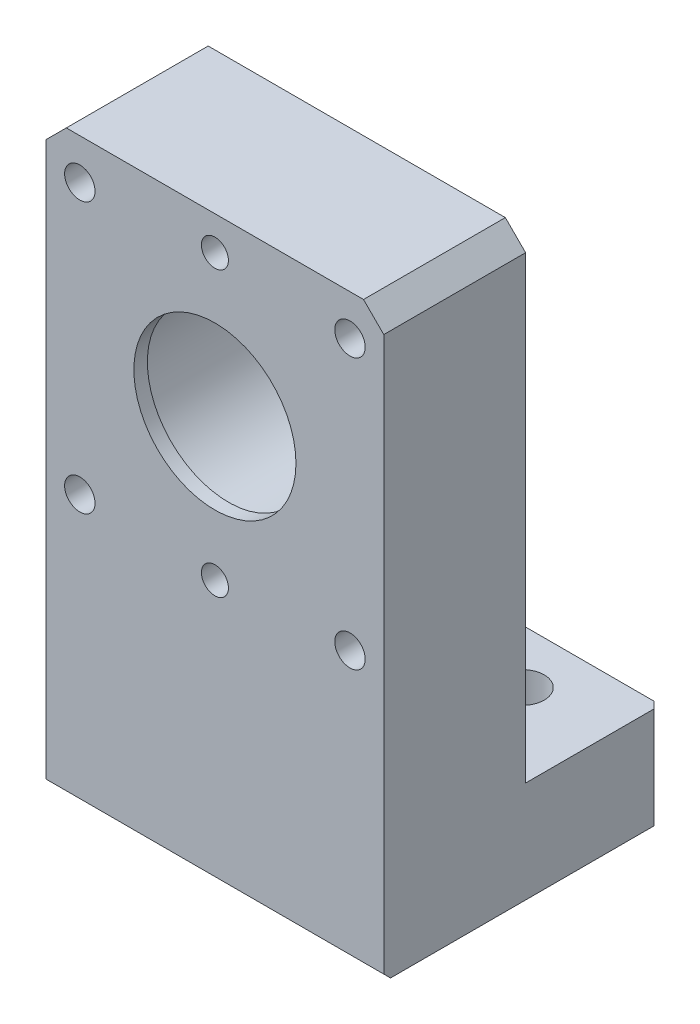
SolidWorks part; units mm, degrees
ref_plane "Front Plane" through (0, 0, 0) normal (0, 0, 1) x (1, 0, 0)
ref_plane "Top Plane" through (0, 0, 0) normal (0, 1, 0) x (1, 0, 0)
ref_plane "Right Plane" through (0, 0, 0) normal (1, 0, 0) x (0, 0, -1)
sketch "Sketch3" plane through (0, 0, 0) normal (0, 0, 1) x (1, 0, 0)
  line L1 (25, 0) -> (-25, 0)
  line L2 (25, 0) -> (25, 86)
  line L3 (25, 86) -> (-25, 86)
  line L4 (-25, 0) -> (-25, 86)
  circle A0 centre (0, 60) radius 14
  dimension "D3" = 28
  dimension "D4" = 60
  dimension "D1" = 50
  dimension "D2" = 86
extrude "Boss-Extrude1" add sketch "Sketch3" along normal blind 21
sketch "Sketch4" plane through (0, 0, 21) normal (0, 0, 1) x (1, 0, 0)
  circle A0 centre (0, 60) radius 14
  circle A1 centre (0, 60) radius 12
  dimension "D1" = 28
  dimension "D2" = 24
hole_wizard "M3 Tapped Hole1" positions "Sketch7" profile "Sketch6" tap size "M3" standard "GB"
sketch "Sketch7" plane through (6.3989, 17.9257, 0) normal (0, 0, 1) x (1, 0, 0)
  line L2 (-6.3989, 42.0743) -> (11.6011, 42.0743) construction
  line L4 (-6.3989, 42.0743) -> (-24.3989, 42.0743) construction
  point P0 (11.6011, 42.0743)
  point P1 (-24.3989, 42.0743)
  dimension "D1" = 18
  dimension "D2" = 18
sketch "Sketch6" plane through (18, 60, 0) normal (1, 0, 0) x (0, 1, 0)
  line L0 (0, 0) -> (0, 10.7511)
  line L1 (0, 10.7511) -> (1.25, 10)
  line L2 (1.25, 10) -> (1.25, 0)
  line L5 (1.25, 0) -> (0, 0)
  line L10 (0, 10.7511) -> (-1.25, 10) construction
  line L11 (0, -6.35) -> (0, 107.95) construction
  dimension "螺纹孔钻头直径" = 2.5
  dimension "螺纹孔钻头深度" = 10
  dimension "导头角度" = 118
cosmetic thread "Cosmetic Thread3" parameters "D1"=8, "D2"=3
cosmetic thread "Cosmetic Thread4" parameters "D1"=8, "D2"=3
extrude "Boss-Extrude3" add sketch "Sketch4" against normal blind 2
hole_wizard "Ø4.0 (4) Diameter Hole2" positions "Sketch15" profile "Sketch14" hole size "Ø4.0" standard "Gb" end condition through all
sketch "Sketch15" plane through (0, 0, 21) normal (0, 0, 1) x (1, 0, 0)
  line L0 (0, 81) -> (0, 39) construction
  circle A0 centre (0, 60) radius 21 construction
  point P1 (0, 81)
  point P5 (0, 39)
  dimension "D1" = 42
sketch "Sketch14" plane through (0, 81, 21) normal (1, 0, 0) x (0, -1, 0)
  line L0 (0, 0) -> (0, 21)
  line L1 (0, 21) -> (2, 21)
  line L2 (2, 21) -> (2, 0)
  line L5 (2, 0) -> (0, 0)
  line L11 (0, -6.35) -> (0, 107.95) construction
  dimension "通孔孔直径" = 4
  dimension "通孔孔深度" = 21
sketch "Sketch22" plane through (0, 0, 0) normal (0, 0, -1) x (-1, 0, 0)
  line L0 (25, 86) -> (25, 0) construction
  line L1 (-25, 0) -> (25, 0)
  line L2 (-25, 0) -> (-25, 15)
  line L3 (-25, 15) -> (25, 15)
  line L4 (25, 0) -> (25, 15)
  dimension "D1" = 15
extrude "Boss-Extrude5" add sketch "Sketch22" along normal blind 20
sketch "Sketch23" plane through (0, 0, 0) normal (0, -1, 0) x (1, 0, 0)
  line L0 (25, -20) -> (-25, -20) construction
  circle A0 centre (12.5, -12) radius 3.25
  circle A1 centre (-12.5, -12) radius 3.25
  dimension "D1" = 6.5
  dimension "D2" = 25
  dimension "D4" = 8
  dimension "D3" = 12.5
extrude "Cut-Extrude3" cut sketch "Sketch23" against normal through all
hole_wizard "Ø4.0 (4) Diameter Hole1" positions "Sketch25" profile "Sketch24" hole size "Ø4.0" standard "Gb"
sketch "Sketch25" plane through (0, 0, 0) normal (0, -1, 0) x (1, 0, 0)
  line L0 (25, -20) -> (-25, -20) construction
  point P0 (0, -15)
  point P2 (0, -5)
  dimension "D1" = 10
  dimension "D2" = 5
sketch "Sketch24" plane through (0, 0, -15) normal (1, 0, 0) x (0, 0, -1)
  line L0 (0, 0) -> (0, 16.2017)
  line L1 (0, 16.2017) -> (2, 15)
  line L2 (2, 15) -> (2, 0)
  line L5 (2, 0) -> (0, 0)
  line L10 (0, 16.2017) -> (-2, 15) construction
  line L11 (0, -6.35) -> (0, 107.95) construction
  dimension "孔直径" = 4
  dimension "孔深度" = 15
  dimension "导头角度" = 118
hole_wizard "Hole size per socket head cap screw type 1" positions "Sketch27" profile "Sketch26" counterbore size "M4" standard "Gb" end condition through all
sketch "Sketch27" plane through (0, 0, 0) normal (0, 0, -1) x (-1, 0, 0)
  circle A0 centre (0, 60) radius 12 construction
  circle A1 centre (0, 60) radius 14 construction
  point P0 (-20, 80)
  point P2 (-20, 40)
  point P4 (20, 40)
  point P6 (20, 80)
  dimension "D1" = 40
  dimension "D2" = 40
  dimension "D3" = 20
  dimension "D4" = 20
sketch "Sketch26" plane through (20, 80, 0) normal (1, 0, 0) x (0, 1, 0)
  line L0 (0, 0) -> (0, 21)
  line L1 (0, 21) -> (2.25, 21)
  line L3 (2.25, 21) -> (2.25, 4.6)
  line L4 (2.25, 4.6) -> (4, 4.6)
  line L5 (4, 4.6) -> (4, 0)
  line L7 (4, 0) -> (0, 0)
  line L11 (0, -6.35) -> (0, 107.95) construction
  dimension "通孔孔直径" = 4.5
  dimension "通孔孔深度" = 21
  dimension "柱形沉头孔直径" = 8
  dimension "柱形沉头孔深度" = 4.6
chamfer "Chamfer1" distance 3 angle 45 2 edges at (-25, 86, 10.5) (25, 86, 10.5)
chamfer "Chamfer2" distance 1 angle 45 3 edges at (0, 0, 21) (25, 7.5, -20) (-25, 7.5, -20)
